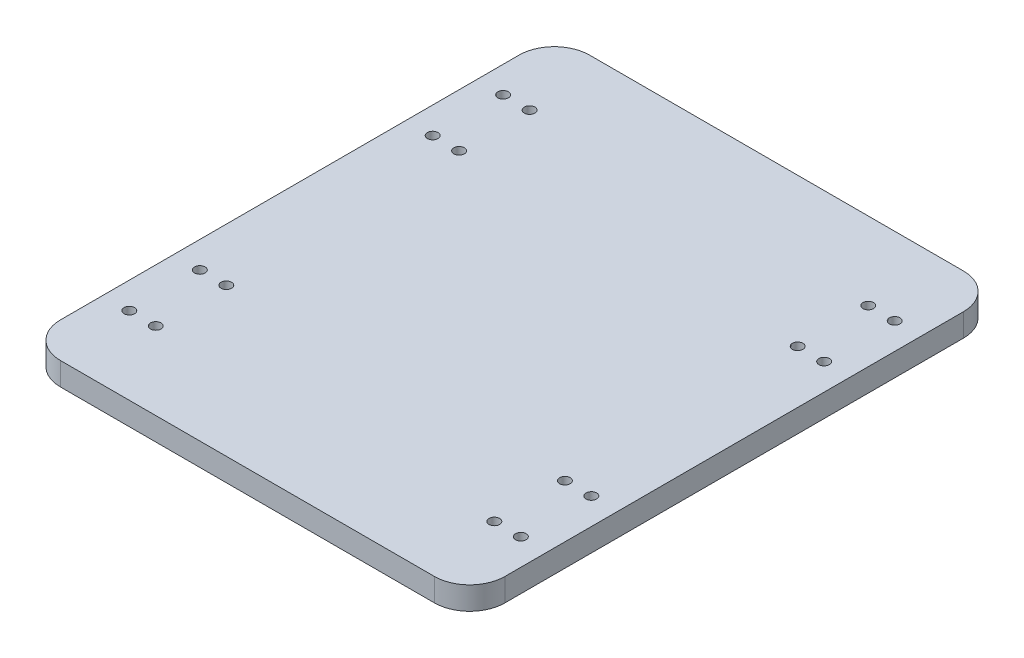
SolidWorks part; units mm, degrees
ref_plane "Front Plane" through (0, 0, 0) normal (0, 0, 1) x (1, 0, 0)
ref_plane "Top Plane" through (0, 0, 0) normal (0, 1, 0) x (1, 0, 0)
ref_plane "Right Plane" through (0, 0, 0) normal (1, 0, 0) x (0, 0, -1)
other "Configuration Table"
sketch "Sketch1" plane through (0, 0, 0) normal (0, 1, 0) x (1, 0, 0)
  line L1 (-63, -75) -> (63, -75)
  line L2 (-63, -75) -> (-63, 75)
  line L3 (-63, 75) -> (63, 75)
  line L4 (63, -75) -> (63, 75)
  line L5 (0, 75) -> (0, -75) construction
  line L6 (-63, 0) -> (63, 0) construction
  point P0 (0, 0)
  dimension "D1" = 126
  dimension "D2" = 150
extrude "Boss-Extrude1" add sketch "Sketch1" along normal blind 6.5
sketch "Sketch2" plane through (0, 6.5, 0) normal (0, 1, 0) x (1, 0, 0)
  line L0 (63, 75) -> (-63, 75) construction
  line L1 (-55.5, 33) -> (-48, 33) construction
  line L2 (-55.5, 33) -> (-55.5, 53) construction
  line L3 (-55.5, 53) -> (-48, 53) construction
  line L4 (-48, 33) -> (-48, 53) construction
  line L5 (-51.75, 53) -> (-51.75, 33) construction
  line L6 (-55.5, 43) -> (-48, 43) construction
  line L7 (-63, 75) -> (-63, -75) construction
  circle A0 centre (-55.5, 33) radius 1.5
  circle A1 centre (-48, 33) radius 1.5
  circle A2 centre (-48, 53) radius 1.5
  circle A3 centre (-55.5, 53) radius 1.5
  point P0 (-51.75, 43)
  dimension "D3" = 3
  dimension "D1" = 20
  dimension "D2" = 7.5
  dimension "D4" = 22
  dimension "D5" = 7.5
extrude "Cut-Extrude1" cut sketch "Sketch2" against normal blind 10
mirror "Mirror1" about plane through (0, 0, 0) normal (1, 0, 0) of "Cut-Extrude1"
mirror "Mirror2" about plane through (0, 0, 0) normal (0, 0, 1) of "Cut-Extrude1", "Mirror1"
fillet "Fillet1" radius 10 4 edges at (63, 3.25, 75) (-63, 3.25, 75) (63, 3.25, -75) (-63, 3.25, -75)
